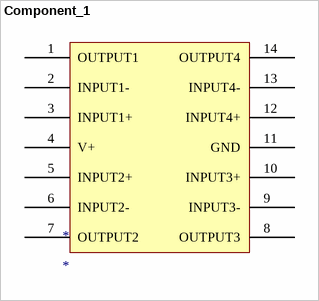
[diagram p0: symbol Component_1]
# Altium schematic symbol library MISC89340-9.SchLib: 1 symbol
Pins are listed as number, name and electrical type; pins without a type are passive.


## Component_1
designator *
footprint LM324
pins: 1 OUTPUT1, 2 INPUT1-, 3 INPUT1+, 4 V+, 5 INPUT2+, 6 INPUT2-, 7 OUTPUT2, 8 OUTPUT3, 9 INPUT3-, 10 INPUT3+, 11 GND, 12 INPUT4+, 13 INPUT4-, 14 OUTPUT4